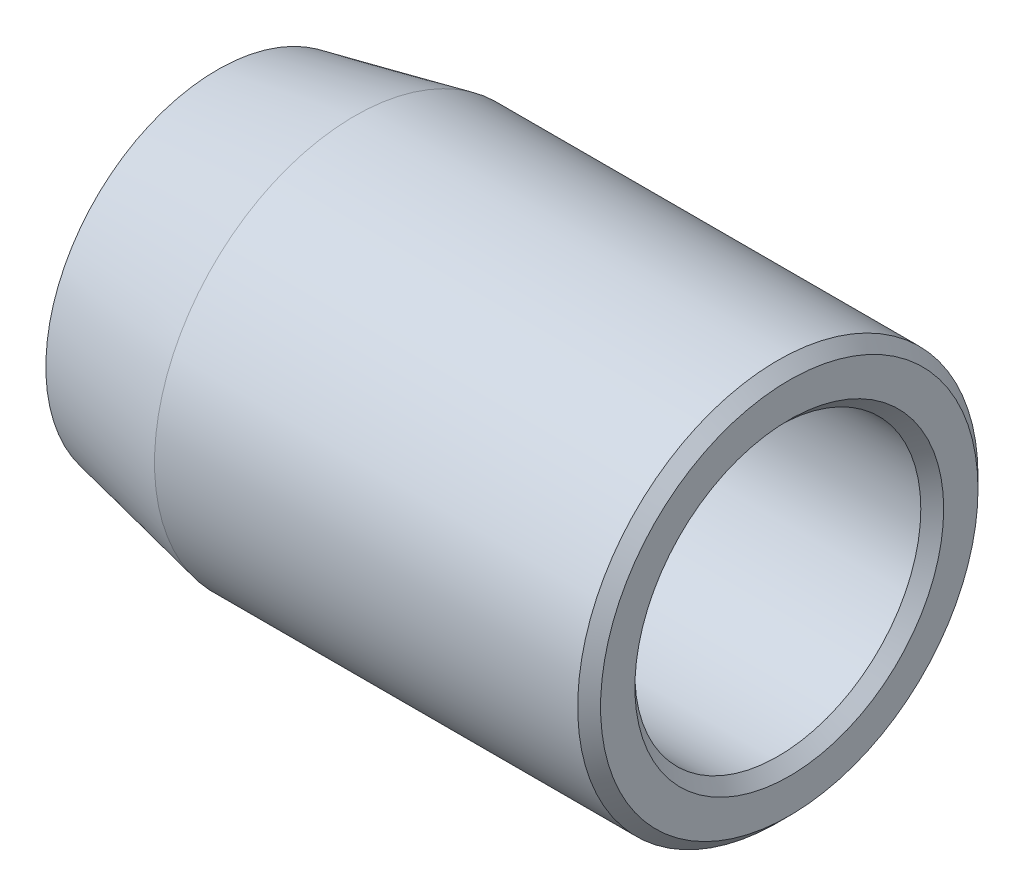
from build123d import *

# Parameters (mm, degrees)
CHAMFER1_SIZE = 1


with BuildPart() as part:
    # Sketch1 → Revolve1 (revolve)
    with BuildSketch(Plane.XY, mode=Mode.PRIVATE) as revolve1_sk:
        Polygon((0, 12.5), (0, 17.5), (-38, 17.5), (-50, 15), (-50, 12.5), align=None)
    revolve(revolve1_sk.sketch.rotate(Axis((0, 0, 0), (-1, 0, 0)), 90), axis=Axis((0, 0, 0), (-1, 0, 0)))

    # Chamfer1
    chamfer1_edges = [part.edges().sort_by_distance(p)[0] for p in [
        (0, 0, 17.5),
        (0, 0, 12.5),
    ]]
    chamfer(chamfer1_edges, length=CHAMFER1_SIZE)


solid = part.part
